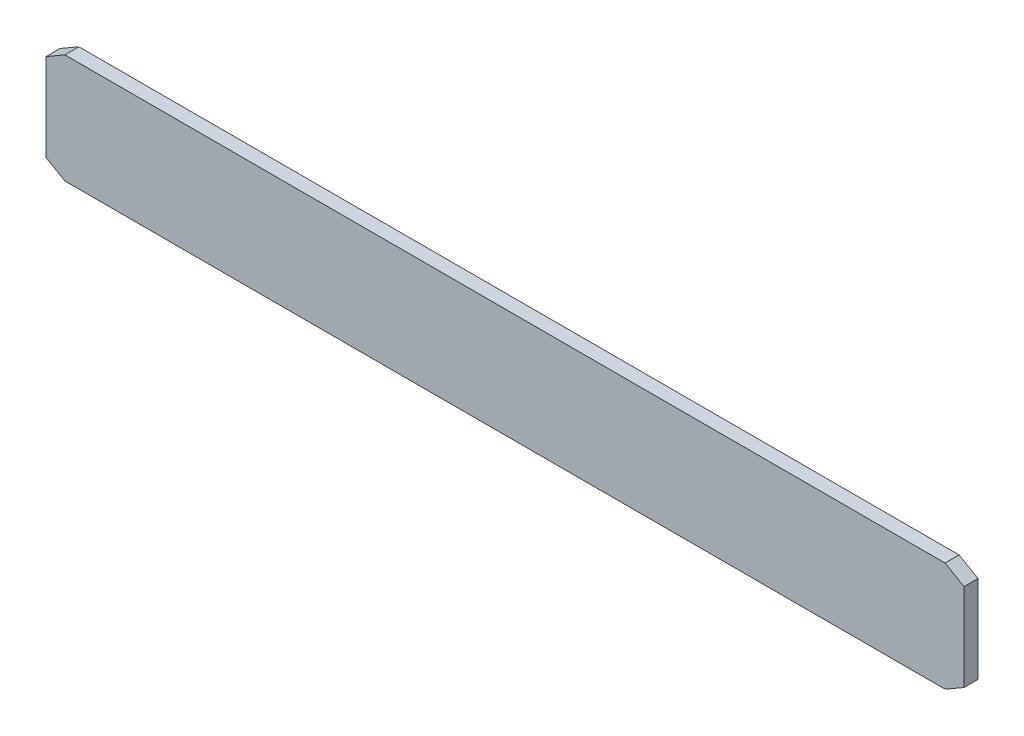
SolidWorks part; units mm, degrees
material "Q235"
ref_plane "Front Plane" through (0, 0, 0) normal (0, 0, 1) x (1, 0, 0)
ref_plane "Top Plane" through (0, 0, 0) normal (0, 1, 0) x (1, 0, 0)
ref_plane "Right Plane" through (0, 0, 0) normal (1, 0, 0) x (0, 0, -1)
sketch "Sketch1" plane through (0, 0, 0) normal (0, 0, 1) x (1, 0, 0)
  line L0 (1050, 100) -> (1006.6987, 125)
  line L1 (-1006.6987, 125) -> (1006.6987, 125)
  line L2 (-1050, 100) -> (-1050, -100)
  line L3 (-1006.6987, -125) -> (1006.6987, -125)
  line L4 (1050, 100) -> (1050, -100)
  line L5 (-1626.1669, 0) -> (1772.2188, 0) construction
  line L6 (1050, -100) -> (1006.6987, -125)
  line L7 (0, 767.823) -> (0, -407.5973) construction
  line L8 (-1050, -100) -> (-1006.6987, -125)
  line L9 (-1050, 100) -> (-1006.6987, 125)
  dimension "D2" = 125
  dimension "D3" = 2100
  dimension "D5" = 100
  dimension "D6" = 30
extrude "Boss-Extrude1" add sketch "Sketch1" along normal mid plane 32
